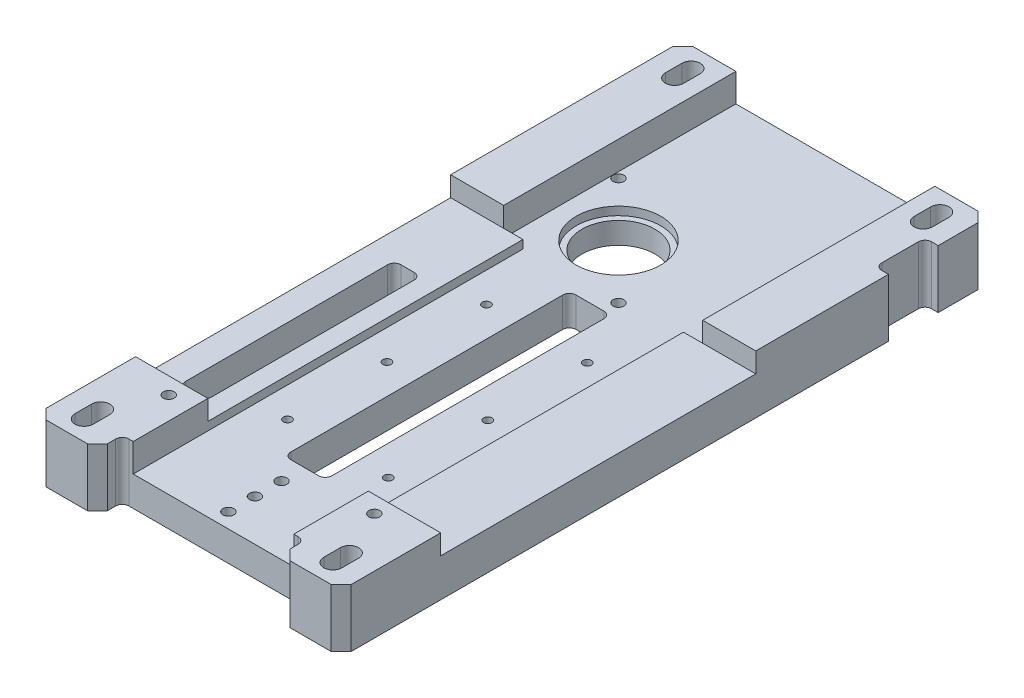
SolidWorks part; units mm, degrees
ref_plane "Front Plane" through (0, 0, 0) normal (0, 0, 1) x (1, 0, 0)
ref_plane "Top Plane" through (0, 0, 0) normal (0, 1, 0) x (1, 0, 0)
ref_plane "Right Plane" through (0, 0, 0) normal (1, 0, 0) x (0, 0, -1)
sketch "Sketch1" plane through (0, 0, 0) normal (0, 1, 0) x (1, 0, 0)
  line L1 (-46, 115) -> (46, 115)
  line L2 (-46, 115) -> (-46, -115)
  line L3 (-46, -115) -> (46, -115)
  line L4 (46, 115) -> (46, -115)
  line L5 (-46, 115) -> (46, -115) construction
  line L6 (-46, -115) -> (46, 115) construction
  point P0 (0, 0)
  dimension "D1" = 92
  dimension "D2" = 230
extrude "Boss-Extrude1" add sketch "Sketch1" along normal blind 17.5
sketch "Sketch3" plane through (0, 0, 0) normal (0, -1, 0) x (1, 0, 0)
  line L0 (-46, -115) -> (-46, 115) construction
  line L1 (46, -115) -> (-46, -115)
  line L2 (46, -115) -> (46, -95)
  line L3 (46, -95) -> (-46, -95)
  line L4 (-46, -115) -> (-46, -95)
  dimension "D1" = 20
extrude "Cut-Extrude2" cut sketch "Sketch3" against normal blind 57
sketch "Sketch7" plane through (0, 0, 0) normal (0, -1, 0) x (1, 0, 0)
  line L0 (-46, -95) -> (-46, 115) construction
  line L1 (46, -95) -> (-46, -95)
  line L2 (46, -95) -> (46, -60)
  line L3 (46, -60) -> (-46, -60)
  line L4 (-46, -95) -> (-46, -60)
  dimension "D1" = 35
extrude "Cut-Extrude5" cut sketch "Sketch7" against normal blind 70
sketch "Sketch6" plane through (0, 17.5, 0) normal (0, 1, 0) x (1, 0, 0)
  line L0 (-24.2, 60) -> (24.2, 60)
  line L1 (0, 0) -> (0, 50000) construction
  line L2 (24.2, 60) -> (24.2, -115)
  line L3 (24.2, -115) -> (-24.2, -115)
  line L4 (-24.2, 60) -> (-24.2, -115)
  line L5 (0, 0) -> (-24.2, -115) construction
  line L6 (24.2, -115) -> (0, 0) construction
  line L7 (-46, 60) -> (46, 60) construction
  line L8 (46, -115) -> (46, 60) construction
  line L9 (-46, 60) -> (-46, -115) construction
  line L10 (-46, -115) -> (46, -115) construction
  point P0 (0, 0)
  dimension "D1" = 48.4
  dimension "D2" = 0
extrude "Cut-Extrude4" cut sketch "Sketch6" against normal blind 8.5
hole_wizard "M3 Tapped Hole1" positions "Sketch9" profile "Sketch10" tap size "M3" standard "Gb" end condition through all
sketch "Sketch9" plane through (0, 9, 0) normal (0, 1, 0) x (1, 0, 0)
  line L0 (0, -115) -> (0, 49885) construction
  line L1 (-24.2, -115) -> (24.2, -115) construction
  point P0 (15.2, -90)
  point P3 (-15.2, -90)
  point P6 (-15.2, -60)
  point P9 (15.2, -60)
  point P12 (15.2, -30)
  point P15 (-15.2, -30)
  point P28 (0, -115)
  dimension "D1" = 30.4
  dimension "D2" = 25
  dimension "D3" = 30
  dimension "D4" = 30
sketch "Sketch10" plane through (15.2, 9, 90) normal (1, 0, 0) x (0, 0, 1)
  line L0 (0, 0) -> (0, 9)
  line L1 (0, 9) -> (1.25, 9)
  line L2 (1.25, 9) -> (1.25, 0)
  line L5 (1.25, 0) -> (0, 0)
  line L11 (0, -6.35) -> (0, 107.95) construction
  dimension "通孔螺纹孔钻头直径" = 2.5
  dimension "通孔螺纹孔钻头深度" = 9
cosmetic thread "Cosmetic Thread1" parameters "D2"=3
cosmetic thread "Cosmetic Thread2" parameters "D2"=3
cosmetic thread "Cosmetic Thread3" parameters "D2"=3
cosmetic thread "Cosmetic Thread4" parameters "D2"=3
cosmetic thread "Cosmetic Thread5" parameters "D2"=3
cosmetic thread "Cosmetic Thread6" parameters "D2"=3
sketch "Sketch4" plane through (0, 0, 0) normal (0, -1, 0) x (1, 0, 0)
  line L0 (0, 0) -> (0, -50000) construction
  line L1 (-46, 115) -> (46, 115) construction
  line L2 (-6.2, 14) -> (6.2, 14)
  line L3 (-6.2, 14) -> (-6.2, 100)
  line L4 (-6.2, 100) -> (6.2, 100)
  line L5 (6.2, 14) -> (6.2, 100)
  line L6 (-6.2, 14) -> (6.2, 100) construction
  line L7 (-6.2, 100) -> (6.2, 14) construction
  point P3 (0, 57)
  dimension "D1" = 12.4
  dimension "D2" = 15
  dimension "D3" = 86
extrude "Cut-Extrude3" cut sketch "Sketch4" against normal blind 29
chamfer "Chamfer1" distance 3 angle 45 2 edges at (-46, 8.75, -60) (46, 8.75, -60)
fillet "Fillet1" radius 2 4 edges at (-6.2, 4.5, 100) (6.2, 4.5, 100) (6.2, 4.5, 14) (-6.2, 4.5, 14)
sketch "Sketch2" plane through (0, 0, 0) normal (0, -1, 0) x (1, 0, 0)
  line L0 (0, 0) -> (0, -50000) construction
  line L1 (43, -60) -> (-43, -60) construction
  line L3 (46, 115) -> (46, -57) construction
  circle A0 centre (-12, -6.6) radius 11
  dimension "D1" = 22
  dimension "D2" = 53.4
  dimension "D3" = 58
extrude "Cut-Extrude1" cut sketch "Sketch2" against normal blind 10
sketch "Sketch20" plane through (0, 0, 115) normal (0, 0, 1) x (1, 0, 0)
  line L0 (-46, 17.5) -> (-24.2, 17.5) construction
  line L1 (-46, 17.5) -> (-46, 0) construction
  line L2 (-24.2, 9) -> (-24.2, 17.5) construction
  line L3 (24.2, 9) -> (-24.2, 9) construction
  line L4 (-46, 0) -> (46, 0) construction
  line L5 (24.2, 17.5) -> (46, 17.5) construction
  line L6 (46, 17.5) -> (46, 0) construction
  line L7 (24.2, 17.5) -> (24.2, 9) construction
  line L8 (-46, 17.5) -> (-24.2, 17.5)
  line L9 (-46, 17.5) -> (-46, 0)
  line L10 (-24.2, 9) -> (-24.2, 17.5)
  line L11 (24.2, 9) -> (-24.2, 9)
  line L12 (-46, 0) -> (46, 0)
  line L13 (24.2, 17.5) -> (46, 17.5)
  line L14 (46, 17.5) -> (46, 0)
  line L15 (24.2, 17.5) -> (24.2, 9)
extrude "Boss-Extrude2" add sketch "Sketch20" along normal blind 20
sketch "Sketch21" plane through (0, 0, 0) normal (0, -1, 0) x (1, 0, 0)
  line L0 (-37.5, 129) -> (-37.5, 124) construction
  line L1 (-34.75, 129) -> (-34.75, 124)
  line L2 (-40.25, 129) -> (-40.25, 124)
  line L3 (0, 125) -> (0, -49875) construction
  line L4 (-46, 135) -> (46, 135) construction
  line L5 (-46, 37.5) -> (49954, 37.5) construction
  line L7 (37.5, 129) -> (37.5, 124) construction
  line L8 (34.75, 129) -> (34.75, 124)
  line L9 (40.25, 129) -> (40.25, 124)
  line L10 (37.5, -54) -> (37.5, -49) construction
  line L11 (34.75, -54) -> (34.75, -49)
  line L12 (40.25, -54) -> (40.25, -49)
  line L13 (-37.5, -54) -> (-37.5, -49) construction
  line L14 (-34.75, -54) -> (-34.75, -49)
  line L15 (-40.25, -54) -> (-40.25, -49)
  line L17 (43, -60) -> (-43, -60) construction
  arc A0 (-34.75, 129) -> (-40.25, 129) centre (-37.5, 129) ccw
  arc A1 (-40.25, 124) -> (-34.75, 124) centre (-37.5, 124) ccw
  arc A2 (34.75, 129) -> (40.25, 129) centre (37.5, 129) cw
  arc A3 (40.25, 124) -> (34.75, 124) centre (37.5, 124) cw
  arc A4 (34.75, -54) -> (40.25, -54) centre (37.5, -54) ccw
  arc A5 (40.25, -49) -> (34.75, -49) centre (37.5, -49) ccw
  arc A6 (-34.75, -54) -> (-40.25, -54) centre (-37.5, -54) cw
  arc A7 (-40.25, -49) -> (-34.75, -49) centre (-37.5, -49) cw
  point P2 (-37.5, 126.5)
  point P11 (0, 135)
  point P19 (37.5, 126.5)
  point P26 (37.5, -51.5)
  point P33 (-37.5, -51.5)
  dimension "D1" = 5.5
  dimension "D2" = 178
  dimension "D3" = 75
  dimension "D4" = 5
extrude "Cut-Extrude9" cut sketch "Sketch21" against normal through all
chamfer "Chamfer2" distance 3 angle 45 2 edges at (-46, 8.75, 135) (46, 8.75, 135)
sketch "Sketch22" plane through (0, 0, 0) normal (0, -1, 0) x (1, 0, 0)
  line L0 (-46, -57) -> (-46, 132) construction
  line L1 (-38, 100) -> (-30, 100)
  line L2 (-38, 100) -> (-38, 35)
  line L3 (-38, 35) -> (-30, 35)
  line L4 (-30, 100) -> (-30, 35)
  line L5 (-43, 135) -> (43, 135) construction
  dimension "D1" = 8
  dimension "D2" = 65
  dimension "D3" = 8
  dimension "D4" = 35
extrude "Cut-Extrude10" cut sketch "Sketch22" against normal through all
fillet "Fillet2" radius 2 4 edges at (-30, 8.75, 100) (-38, 8.75, 100) (-38, 8.75, 35) (-30, 8.75, 35)
sketch "Sketch12" plane through (0, 9, 0) normal (0, 1, 0) x (1, 0, 0)
  circle A0 centre (-12, 6.6) radius 12.75
  dimension "D1" = 25.5
extrude "Cut-Extrude7" cut sketch "Sketch12" against normal blind 2.5
sketch "Sketch23" plane through (0, 17.5, 0) normal (0, 1, 0) x (1, 0, 0)
  line L0 (-12, 3) -> (-12, 50003) construction
  line L1 (-46, 57) -> (-46, -132) construction
  line L2 (-46, -10) -> (46, -10)
  line L3 (-46, -10) -> (-46, -105)
  line L4 (-46, -105) -> (46, -105)
  line L5 (46, -10) -> (46, -105)
  line L6 (46, -132) -> (46, 57) construction
  line L7 (24.2, 60) -> (-24.2, 60) construction
  line L8 (43, -135) -> (24.2, -135) construction
  dimension "D1" = 70
  dimension "D2" = 30
extrude "Cut-Extrude11" cut sketch "Sketch23" against normal blind 6
hole_wizard "M2.5 Tapped Hole1" positions "3DSketch4" profile "Sketch24" tap size "M2.5" standard "Gb"
sketch3d "3DSketch4"
  point P0 (-10.2, 0, 83.8915)
  point P2 (-10.2, 0, 70.8915)
  dimension "D1" = 4
  dimension "D2" = 13
  dimension "D3" = 51.1085
sketch "Sketch24" plane through (-10.2, 0, 83.8915) normal (1, 0, 0) x (0, 0, -1)
  line L0 (0, 0) -> (0, 6.9659)
  line L1 (0, 6.9659) -> (1.025, 6.35)
  line L2 (1.025, 6.35) -> (1.025, 0)
  line L5 (1.025, 0) -> (0, 0)
  line L10 (0, 6.9659) -> (-1.025, 6.35) construction
  line L11 (0, -6.35) -> (0, 107.95) construction
  dimension "螺纹孔钻头直径" = 2.05
  dimension "螺纹孔钻头深度" = 6.35
  dimension "导头角度" = 118
cosmetic thread "Cosmetic Thread11" parameters "D1"=5, "D2"=2.5
cosmetic thread "Cosmetic Thread12" parameters "D1"=5, "D2"=2.5
hole_wizard "M4 Tapped Hole3" positions "3DSketch5" profile "Sketch26" tap size "M4" standard "Gb"
sketch3d "3DSketch5"
  line L0 (-46, 0, -57) -> (-46, 0, 132) construction
  point P0 (0, 0, 107)
  dimension "D1" = 46
  dimension "D2" = 28
sketch "Sketch26" plane through (0, 0, 107) normal (1, 0, 0) x (0, 0, -1)
  line L0 (0, 0) -> (0, 11.0914)
  line L1 (0, 11.0914) -> (1.65, 10.1)
  line L2 (1.65, 10.1) -> (1.65, 0)
  line L5 (1.65, 0) -> (0, 0)
  line L10 (0, 11.0914) -> (-1.65, 10.1) construction
  line L11 (0, -6.35) -> (0, 107.95) construction
  dimension "螺纹孔钻头直径" = 3.3
  dimension "螺纹孔钻头深度" = 10.1
  dimension "导头角度" = 118
cosmetic thread "Cosmetic Thread13" parameters "D1"=8, "D2"=4
hole_wizard "M4 Tapped Hole4" positions "Sketch28" profile "Sketch27" tap size "M4" standard "Gb"
sketch "Sketch28" plane through (0, 17.5, 0) normal (0, 1, 0) x (1, 0, 0)
  line L0 (46, -132) -> (46, -105) construction
  line L1 (-46, -105) -> (-46, -132) construction
  line L2 (-24.2, -135) -> (-43, -135) construction
  point P0 (31, -110)
  point P2 (-31, -110)
  dimension "D1" = 15
  dimension "D2" = 15
  dimension "D3" = 25
sketch "Sketch27" plane through (31, 17.5, 110) normal (1, 0, 0) x (0, 0, 1)
  line L0 (0, 0) -> (0, 11.0914)
  line L1 (0, 11.0914) -> (1.65, 10.1)
  line L2 (1.65, 10.1) -> (1.65, 0)
  line L5 (1.65, 0) -> (0, 0)
  line L10 (0, 11.0914) -> (-1.65, 10.1) construction
  line L11 (0, -6.35) -> (0, 107.95) construction
  dimension "螺纹孔钻头直径" = 3.3
  dimension "螺纹孔钻头深度" = 10.1
  dimension "导头角度" = 118
cosmetic thread "Cosmetic Thread14" parameters "D1"=8, "D2"=4
cosmetic thread "Cosmetic Thread15" parameters "D1"=8, "D2"=4
sketch "Sketch16" plane through (0, 0, 0) normal (0, -1, 0) x (1, 0, 0)
  line L0 (0, -6.6) -> (50000, -6.6) construction
  line L1 (-4.2, 1.2) -> (35351.1391, 35356.5391) construction
  circle A0 centre (-12, -6.6) radius 23 construction
  circle A1 centre (4.2635, 9.6635) radius 1
  circle A2 centre (-28.2635, -22.8635) radius 1
  dimension "D1" = 45
  dimension "D2" = 2
  dimension "D3" = 46
extrude "Cut-Extrude8" cut sketch "Sketch16" against normal blind 10
sketch "Sketch30" plane through (0, 0, 0) normal (0, -1, 0) x (1, 0, 0)
  line L0 (46, 132) -> (46, -57) construction
  line L1 (46, -30) -> (42, -30)
  line L2 (46, -30) -> (46, -45)
  line L3 (46, -45) -> (42, -45)
  line L4 (42, -30) -> (42, -45)
  line L5 (43, -60) -> (-43, -60) construction
  dimension "D1" = 4
  dimension "D2" = 15
  dimension "D3" = 15
extrude "Cut-Extrude12" cut sketch "Sketch30" against normal through all
hole_wizard "M4 Tapped Hole2" positions "3DSketch3" profile "Sketch18" tap size "M4" standard "Gb" end condition through all
sketch3d "3DSketch3"
  line L0 (-28.2635, 10, -22.8635) -> (-28.2635, 0, -22.8635) construction
  line L1 (4.2635, 9, 9.6635) -> (4.2635, 0, 9.6635) construction
  point P0 (-28.2635, 0, -22.8635)
  point P4 (4.2635, 0, 9.6635)
sketch "Sketch18" plane through (-28.2635, 0, -22.8635) normal (1, 0, 0) x (0, 0, -1)
  line L0 (0, 0) -> (0, 17.5)
  line L1 (0, 17.5) -> (1.65, 17.5)
  line L2 (1.65, 17.5) -> (1.65, 0)
  line L5 (1.65, 0) -> (0, 0)
  line L11 (0, -6.35) -> (0, 107.95) construction
  dimension "通孔螺纹孔钻头直径" = 3.3
  dimension "通孔螺纹孔钻头深度" = 17.5
cosmetic thread "Cosmetic Thread9" parameters "D2"=4
cosmetic thread "Cosmetic Thread10" parameters "D2"=4
fillet "Fillet3" radius 2 2 edges at (42, 8.75, -45) (42, 8.75, -30)
pattern_linear "LPattern1" count 3 spacing 8 along (0, 0, 1) of "M4 Tapped Hole3"
sketch "Sketch31" plane through (0, 0, 0) normal (0, -1, 0) x (1, 0, 0)
  line L0 (-43, 135) -> (43, 135) construction
  line L1 (-27.5, 142.5) -> (27.5, 142.5)
  line L2 (-27.5, 142.5) -> (-27.5, 127.5)
  line L3 (-27.5, 127.5) -> (27.5, 127.5)
  line L4 (27.5, 142.5) -> (27.5, 127.5)
  line L5 (-27.5, 142.5) -> (27.5, 127.5) construction
  line L6 (-27.5, 127.5) -> (27.5, 142.5) construction
  point P0 (0, 135)
  dimension "D1" = 55
  dimension "D2" = 7.5
extrude "Cut-Extrude13" cut sketch "Sketch31" against normal blind 27
fillet "Fillet4" radius 2 2 edges at (27.5, 8.75, 127.5) (-27.5, 8.75, 127.5)
chamfer "Chamfer3" distance 3 angle 45 2 edges at (-27.5, 8.75, 135) (27.5, 8.75, 135)
sketch "Sketch32" plane through (0, 17.5, 0) normal (0, 1, 0) x (1, 0, 0)
  line L0 (-24.2, -10) -> (-46, -10) construction
  line L1 (-24.2, 60) -> (-30, 60)
  line L2 (-24.2, 60) -> (-24.2, -10)
  line L3 (-24.2, -10) -> (-30, -10)
  line L4 (-30, 60) -> (-30, -10)
  line L5 (0, 60) -> (0, -49940) construction
  line L6 (24.2, 60) -> (-24.2, 60) construction
  line L7 (30, 60) -> (30, -10)
  line L8 (24.2, -10) -> (30, -10)
  line L9 (24.2, 60) -> (24.2, -10)
  line L10 (24.2, 60) -> (30, 60)
  point P11 (0, 60)
  dimension "D1" = 60
extrude "Cut-Extrude14" cut sketch "Sketch32" against normal up to surface (8.5 mm away) up to face at (0, 9, 121.35)
hole_wizard "M3 Tapped Hole2" positions "Sketch34" profile "Sketch33" tap size "M3" standard "Gb"
sketch "Sketch34" plane through (0, 0, 0) normal (0, -1, 0) x (-1, 0, 0)
  line L0 (46, 57) -> (46, -132) construction
  line L1 (-43, 60) -> (43, 60) construction
  point P0 (41, -22)
  dimension "D1" = 5
  dimension "D2" = 82
sketch "Sketch33" plane through (-41, 0, 22) normal (1, 0, 0) x (0, 0, -1)
  line L0 (0, 0) -> (0, 8.2511)
  line L1 (0, 8.2511) -> (1.25, 7.5)
  line L2 (1.25, 7.5) -> (1.25, 0)
  line L5 (1.25, 0) -> (0, 0)
  line L10 (0, 8.2511) -> (-1.25, 7.5) construction
  line L11 (0, -6.35) -> (0, 107.95) construction
  dimension "螺纹孔钻头直径" = 2.5
  dimension "螺纹孔钻头深度" = 7.5
  dimension "导头角度" = 118
cosmetic thread "Cosmetic Thread16" parameters "D1"=6, "D2"=3
hole_wizard "M3 Tapped Hole3" positions "Sketch36" profile "Sketch35" tap size "M3" standard "Gb"
sketch "Sketch36" plane through (0, 0, 0) normal (0, -1, 0) x (-1, 0, 0)
  line L0 (46, 57) -> (46, -132) construction
  line L1 (43, -135) -> (30.5, -135) construction
  point P0 (24, -113)
  dimension "D1" = 22
  dimension "D2" = 22
sketch "Sketch35" plane through (-24, 0, 113) normal (1, 0, 0) x (0, 0, -1)
  line L0 (0, 0) -> (0, 8.2511)
  line L1 (0, 8.2511) -> (1.25, 7.5)
  line L2 (1.25, 7.5) -> (1.25, 0)
  line L5 (1.25, 0) -> (0, 0)
  line L10 (0, 8.2511) -> (-1.25, 7.5) construction
  line L11 (0, -6.35) -> (0, 107.95) construction
  dimension "螺纹孔钻头直径" = 2.5
  dimension "螺纹孔钻头深度" = 7.5
  dimension "导头角度" = 118
cosmetic thread "Cosmetic Thread17" parameters "D1"=6, "D2"=3
